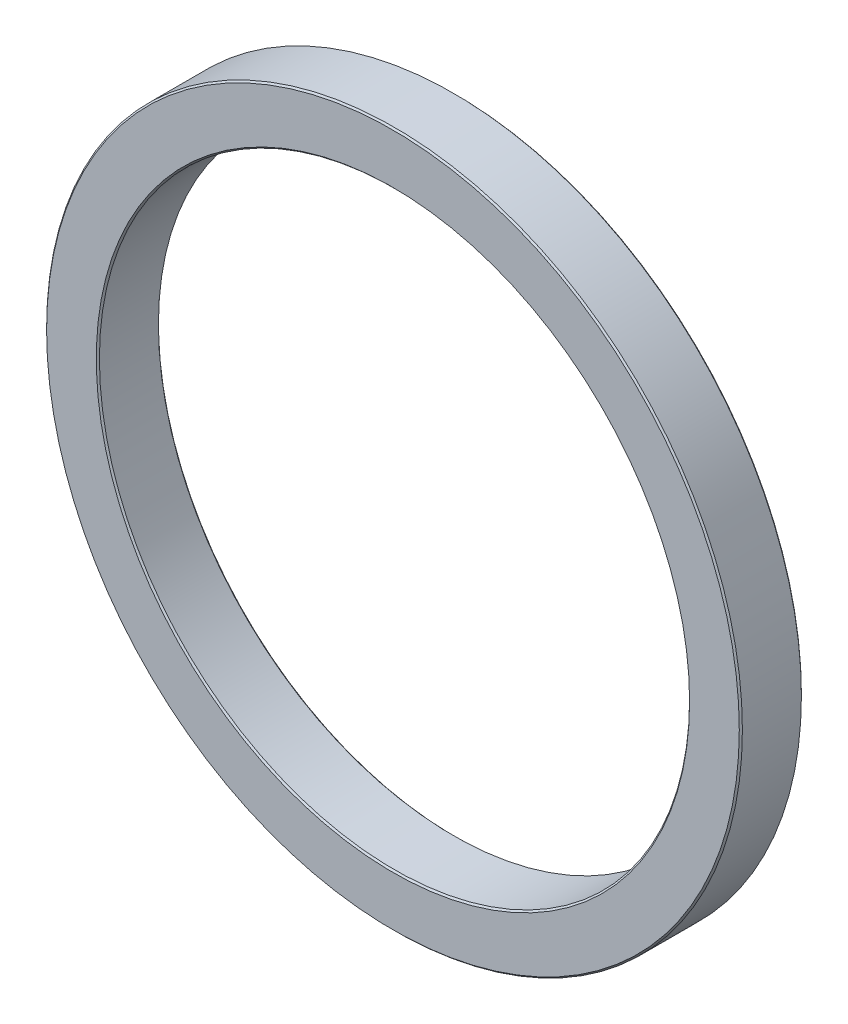
SolidWorks part; units mm, degrees
ref_plane "前视基准面" through (0, 0, 0) normal (0, 0, 1) x (1, 0, 0)
ref_plane "上视基准面" through (0, 0, 0) normal (0, 1, 0) x (1, 0, 0)
ref_plane "右视基准面" through (0, 0, 0) normal (1, 0, 0) x (0, 0, -1)
sketch "草图1" plane through (0, 0, 0) normal (0, 0, 1) x (1, 0, 0)
  circle A0 centre (0, 0) radius 47.5
  circle A1 centre (0, 0) radius 56
  dimension "D1" = 95
  dimension "D2" = 112
extrude "凸台-拉伸1" add sketch "草图1" along normal blind 10
hole_wizard "M4 螺纹孔1" positions "草图4" profile "草图3" tap size "M4" standard "GB"
sketch "草图4" plane through (0, 0, 0) normal (0, 0, -1) x (-1, 0, 0)
  line L0 (0, 0) -> (0, -35.5) construction
  line L3 (0, 0) -> (-34.1455, -34.1455) construction
  line L6 (0, 0) -> (-23.6627, 0) construction
  circle A0 centre (0, 0) radius 53 construction
  point P0 (35.5, 0)
  point P3 (0, 35.5)
  point P6 (0, -35.5)
  point P10 (-35.5, 0)
  point P35 (-37.4767, -37.4767)
  point P39 (37.4767, -37.4767)
  point P40 (37.4767, 37.4767)
  point P41 (-37.4767, 37.4767)
  point P43 (0, 53)
  point P45 (53, 0)
  point P47 (0, -53)
  point P49 (-53, 0)
  dimension "D2" = 106
  dimension "D1" = 45
sketch "草图3" plane through (-35.5, 0, 0) normal (1, 0, 0) x (0, 1, 0)
  line L0 (0, 0) -> (0, 7.5)
  line L1 (0, 7.5) -> (1.65, 7.5)
  line L2 (1.65, 7.5) -> (1.65, 0)
  line L5 (1.65, 0) -> (0, 0)
  line L10 (0, 7.5) -> (-1.65, 7.5) construction
  line L11 (0, -6.35) -> (0, 107.95) construction
  dimension "螺纹孔钻头直径" = 3.3
  dimension "螺纹孔钻头深度" = 7.5
  dimension "导头角度" = 180
cosmetic thread "孔螺蚊线1" parameters "D1"=6, "D2"=4
cosmetic thread "孔螺蚊线2" parameters "D1"=6, "D2"=4
cosmetic thread "孔螺蚊线3" parameters "D1"=6, "D2"=4
cosmetic thread "孔螺蚊线4" parameters "D1"=6, "D2"=4
cosmetic thread "孔螺蚊线5" parameters "D1"=6, "D2"=4
cosmetic thread "孔螺蚊线6" parameters "D1"=6, "D2"=4
cosmetic thread "孔螺蚊线7" parameters "D1"=6, "D2"=4
cosmetic thread "孔螺蚊线8" parameters "D1"=6, "D2"=4
chamfer "倒角1" distance 0.25 angle 45 4 edges at (56, 0, 10) (47.5, 0, 10) (56, 0, 0) (47.5, 0, 0)
sketch "草图5" plane through (0, 0, 0) normal (0, 0, -1) x (-1, 0, 0)
  circle A0 centre (0, 0) radius 48.5
  circle A1 centre (0, 0) radius 50
  dimension "D1" = 97
  dimension "D2" = 1.5
extrude "切除-拉伸1" cut sketch "草图5" against normal blind 1.2
